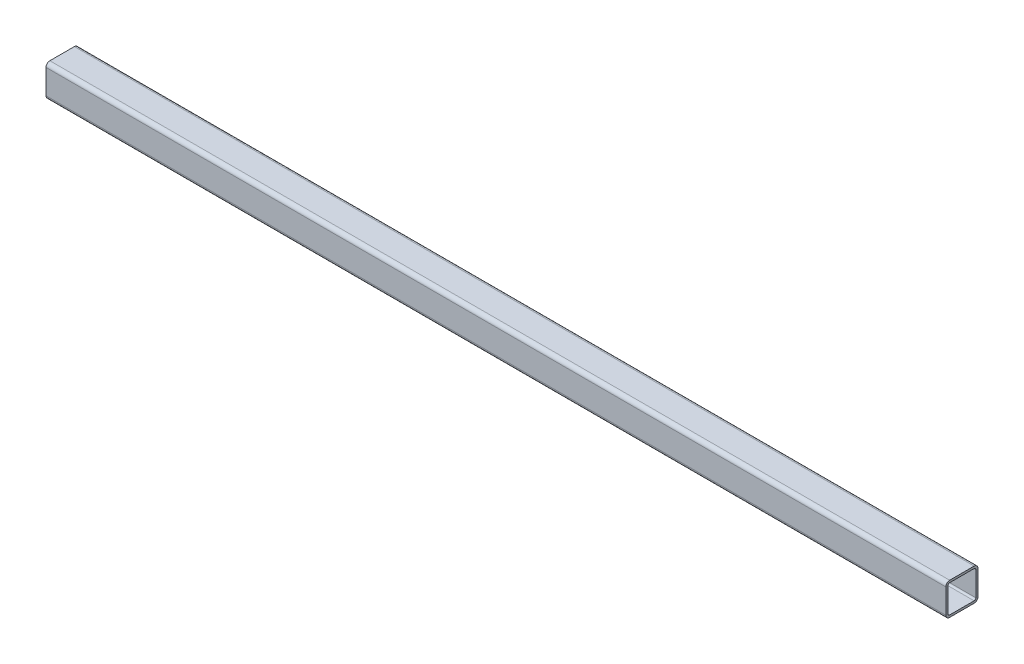
SolidWorks part; units mm, degrees
material "S45C"
ref_plane "前视" through (0, 0, 0) normal (0, 0, 1) x (1, 0, 0)
ref_plane "上视" through (0, 0, 0) normal (0, 1, 0) x (1, 0, 0)
ref_plane "右视" through (0, 0, 0) normal (1, 0, 0) x (0, 0, -1)
sketch "草图1" plane through (0, 0, 0) normal (0, 1, 0) x (1, 0, 0)
  line L0 (-419, 0) -> (419, 0)
  point P4 (0, 0)
  dimension "D1" = 838
other "方管 30×2(1)"
ref_plane "基准面1" through (-419, 0, 0) normal (1, 0, 0) x (0, 0, -1)
sketch "Sketch1" plane through (-419, 0, 0) normal (1, 0, 0) x (0, 0, -1)
  line L0 (-11.4, -13) -> (11.4, -13)
  line L1 (-13, -11.4) -> (-13, 11.4)
  line L2 (11.4, 13) -> (-11.4, 13)
  line L3 (13, 11.4) -> (13, -11.4)
  line L4 (-11.4, -15) -> (11.4, -15)
  line L5 (-15, -11.4) -> (-15, 11.4)
  line L6 (11.4, 15) -> (-11.4, 15)
  line L7 (15, 11.4) -> (15, -11.4)
  arc A0 (15, 11.4) -> (11.4, 15) centre (11.4, 11.4) ccw
  arc A1 (11.4, -15) -> (15, -11.4) centre (11.4, -11.4) ccw
  arc A2 (-15, -11.4) -> (-11.4, -15) centre (-11.4, -11.4) ccw
  arc A3 (-11.4, 15) -> (-15, 11.4) centre (-11.4, 11.4) ccw
  arc A4 (-11.4, 13) -> (-13, 11.4) centre (-11.4, 11.4) ccw
  arc A5 (13, 11.4) -> (11.4, 13) centre (11.4, 11.4) ccw
  arc A6 (11.4, -13) -> (13, -11.4) centre (11.4, -11.4) ccw
  arc A7 (-13, -11.4) -> (-11.4, -13) centre (-11.4, -11.4) ccw
  point P0 (-15, 0)
  point P1 (15, 0)
  point P2 (0, 15)
  point P3 (0, -15)
  point P4 (0, 0)
  point P5 (-15, -15)
  point P6 (15, -15)
  point P7 (15, 15)
  point P8 (-15, 15)
  point P33 (0, 0)
equation "\"D1@Sketch1\" = \"Thickness@Sketch1\"*1.8"
